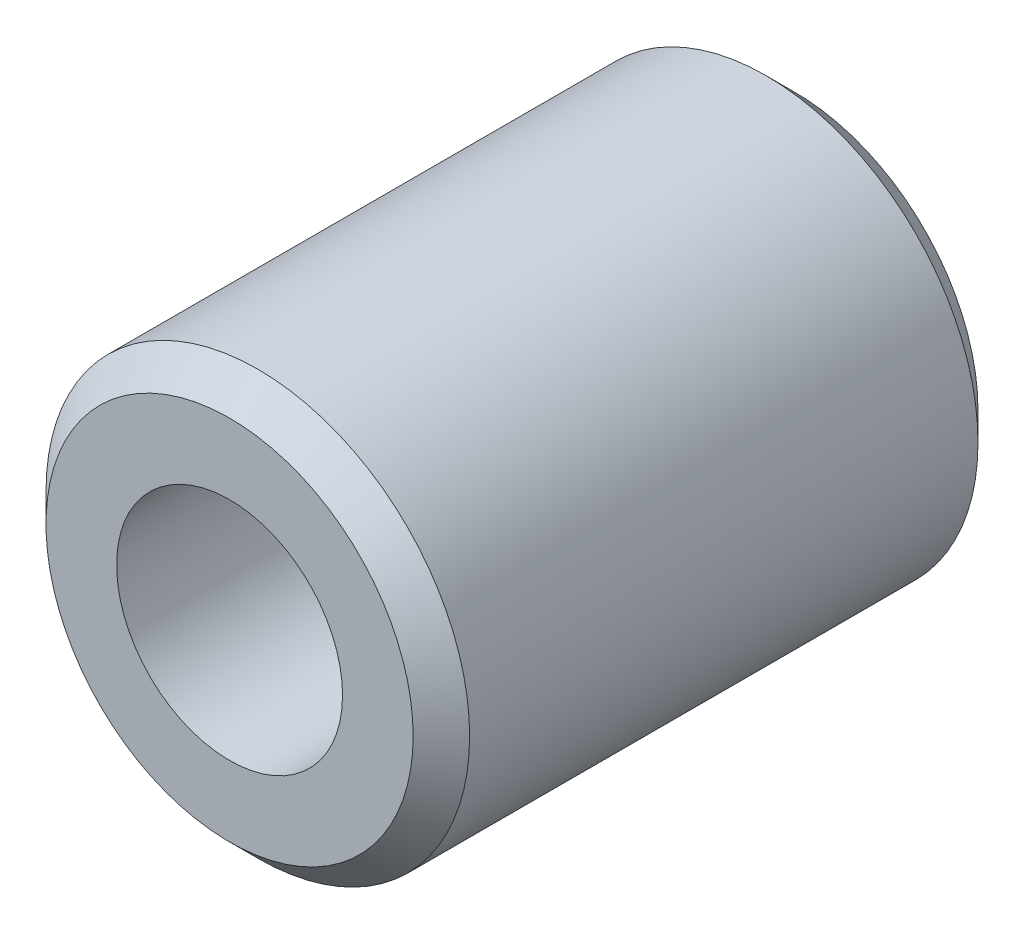
from build123d import *

# Parameters (mm, degrees)
SKETCH1_R           = 7.5
BOSS_EXTRUDE1_DEPTH = 20
CHAMFER1_SIZE       = 1
SKETCH2_R           = 4
CUT_EXTRUDE1_DEPTH  = 20


with BuildPart() as part:
    # Sketch1 → Boss-Extrude1 (new body)
    with BuildSketch(Plane.XY):
        Circle(SKETCH1_R)
    extrude(amount=BOSS_EXTRUDE1_DEPTH)

    # Chamfer1
    chamfer1_edges = [part.edges().sort_by_distance(p)[0] for p in [
        (-7.5, 0, 0),
        (-7.5, 0, 20),
    ]]
    chamfer(chamfer1_edges, length=CHAMFER1_SIZE)

    # Sketch2 → Cut-Extrude1 (cut)
    with BuildSketch(Plane.XY.offset(20)):
        Circle(SKETCH2_R)
    extrude(amount=-CUT_EXTRUDE1_DEPTH, mode=Mode.SUBTRACT)


solid = part.part
